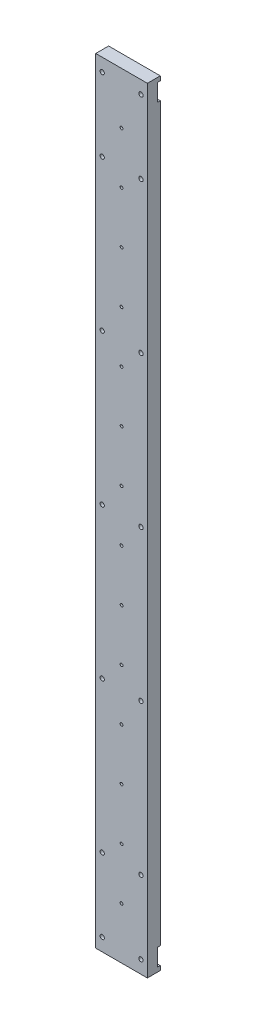
SolidWorks part; units mm, degrees
material "6061 合金"
ref_plane "Front Plane" through (0, 0, 0) normal (0, 0, 1) x (1, 0, 0)
ref_plane "Top Plane" through (0, 0, 0) normal (0, 1, 0) x (1, 0, 0)
ref_plane "Right Plane" through (0, 0, 0) normal (1, 0, 0) x (0, 0, -1)
sketch "Sketch1" plane through (0, 0, 0) normal (0, 0, 1) x (1, 0, 0)
  line L1 (-30, 450) -> (30, 450)
  line L2 (-30, 450) -> (-30, -450)
  line L3 (-30, -450) -> (30, -450)
  line L4 (30, 450) -> (30, -450)
  line L5 (-30, 450) -> (30, -450) construction
  line L6 (-30, -450) -> (30, 450) construction
  point P0 (0, 0)
  dimension "D1" = 60
  dimension "D2" = 900
extrude "Boss-Extrude1" add sketch "Sketch1" along normal blind 15
hole_wizard "CBORE for M6 Hex Socket Head Cap Screw1" positions "Sketch2" profile "Sketch3" counterbore size "M6" standard "ISO"
sketch "Sketch2" plane through (0, 0, 15) normal (0, 0, 1) x (1, 0, 0)
  line L0 (0, 0) -> (176.5363, 0) construction
  point P0 (0, 475)
  point P2 (0, 150)
  point P4 (0, -150)
  point P6 (0, -475)
  dimension "D1" = 300
  dimension "D2" = 950
sketch "Sketch3" plane through (0, 475, 15) normal (1, 0, 0) x (0, -1, 0)
  line L0 (0, 0) -> (0, 15)
  line L1 (0, 15) -> (3.3, 15)
  line L3 (3.3, 15) -> (3.3, 6.4)
  line L4 (3.3, 6.4) -> (5.5, 6.4)
  line L5 (5.5, 6.4) -> (5.5, 0)
  line L7 (5.5, 0) -> (0, 0)
  line L11 (0, -6.35) -> (0, 107.95) construction
  dimension "通孔孔直径" = 6.6
  dimension "通孔孔深度" = 15
  dimension "柱形沉头孔直径" = 11
  dimension "柱形沉头孔深度" = 6.4
sketch "Sketch5" plane through (0, 0, 0) normal (0, 0, -1) x (-1, 0, 0)
  line L0 (-30, -450) -> (-30, 450) construction
  line L1 (-30, 445) -> (30, 445)
  line L2 (-30, 445) -> (-30, 425)
  line L3 (-30, 425) -> (30, 425)
  line L4 (30, 445) -> (30, 425)
  line L5 (30, 450) -> (30, -450) construction
  line L6 (30, -450) -> (-30, -450) construction
  line L7 (-30, -445) -> (30, -445)
  line L8 (-30, -445) -> (-30, -425)
  line L9 (-30, -425) -> (30, -425)
  line L10 (30, -445) -> (30, -425)
  line L11 (-30, 450) -> (30, 450) construction
  dimension "D1" = 20
  dimension "D2" = 5
  dimension "D3" = 5
extrude "Cut-Extrude2" cut sketch "Sketch5" against normal blind 3
sketch "Sketch7" plane through (0, 0, 0) normal (0, 0, -1) x (-1, 0, 0)
  line L0 (-30, 425) -> (30, 425) construction
  line L1 (-7.5, 425) -> (7.5, 425)
  line L2 (-7.5, 425) -> (-7.5, -425)
  line L3 (-7.5, -425) -> (7.5, -425)
  line L4 (7.5, 425) -> (7.5, -425)
  line L5 (30, -425) -> (-30, -425) construction
  dimension "D1" = 15
  dimension "D2" = 7.5
extrude "Cut-Extrude3" cut sketch "Sketch7" against normal blind 2
hole_wizard "M4 Tapped Hole1" positions "Sketch8" profile "Sketch9" tap size "M4" standard "ISO" end condition through all
sketch "Sketch8" plane through (0, 0, 2) normal (0, 0, -1) x (-1, 0, 0)
  line L0 (0, 425) -> (0, 390) construction
  line L1 (7.5, 425) -> (-7.5, 425) construction
  point P0 (0, 390)
  dimension "D1" = 35
sketch "Sketch9" plane through (0, 390, 2) normal (1, 0, 0) x (0, 1, 0)
  line L0 (0, 0) -> (0, 13)
  line L1 (0, 13) -> (1.65, 13)
  line L2 (1.65, 13) -> (1.65, 0)
  line L5 (1.65, 0) -> (0, 0)
  line L11 (0, -6.35) -> (0, 107.95) construction
  dimension "通孔螺纹孔钻头直径" = 3.3
  dimension "通孔螺纹孔钻头深度" = 13
cosmetic thread "Cosmetic Thread1" parameters "D2"=4
pattern_linear "LPattern1" count 14 spacing 60 along (0, -1, 0) of "M4 Tapped Hole1"
cosmetic thread "Cosmetic Thread2" parameters "D2"=4
cosmetic thread "Cosmetic Thread3" parameters "D2"=4
cosmetic thread "Cosmetic Thread4" parameters "D2"=4
cosmetic thread "Cosmetic Thread5" parameters "D2"=4
cosmetic thread "Cosmetic Thread6" parameters "D2"=4
cosmetic thread "Cosmetic Thread7" parameters "D2"=4
cosmetic thread "Cosmetic Thread8" parameters "D2"=4
cosmetic thread "Cosmetic Thread9" parameters "D2"=4
cosmetic thread "Cosmetic Thread10" parameters "D2"=4
cosmetic thread "Cosmetic Thread11" parameters "D2"=4
cosmetic thread "Cosmetic Thread12" parameters "D2"=4
cosmetic thread "Cosmetic Thread13" parameters "D2"=4
cosmetic thread "Cosmetic Thread14" parameters "D2"=4
hole_wizard "M6 Tapped Hole1" positions "Sketch10" profile "Sketch11" tap size "M6" standard "ISO" end condition through all
sketch "Sketch10" plane through (0, 0, 3) normal (0, 0, -1) x (-1, 0, 0)
  line L0 (-30, -435) -> (-22.5, -435) construction
  line L1 (-30, -425) -> (-30, -445) construction
  line L3 (0, -445) -> (0, -434.4677) construction
  line L4 (-30, -445) -> (30, -445) construction
  line L6 (-30, 435) -> (-22.5, 435) construction
  line L7 (-30, 445) -> (-30, 425) construction
  line L9 (0, 445) -> (0, 434.9254) construction
  line L10 (30, 445) -> (-30, 445) construction
  point P0 (-22.5, 435)
  point P2 (22.5, 435)
  point P4 (-22.5, -435)
  point P6 (22.5, -435)
  dimension "D1" = 45
  dimension "D2" = 45
sketch "Sketch11" plane through (22.5, 435, 3) normal (1, 0, 0) x (0, 1, 0)
  line L0 (0, 0) -> (0, 12)
  line L1 (0, 12) -> (2.5, 12)
  line L2 (2.5, 12) -> (2.5, 0)
  line L5 (2.5, 0) -> (0, 0)
  line L11 (0, -6.35) -> (0, 107.95) construction
  dimension "通孔螺纹孔钻头直径" = 5
  dimension "通孔螺纹孔钻头深度" = 12
cosmetic thread "Cosmetic Thread15" parameters "D2"=6
cosmetic thread "Cosmetic Thread16" parameters "D2"=6
cosmetic thread "Cosmetic Thread17" parameters "D2"=6
cosmetic thread "Cosmetic Thread18" parameters "D2"=6
hole_wizard "M6 Tapped Hole2" positions "Sketch12" profile "Sketch13" tap size "M6" standard "ISO" end condition through all
sketch "Sketch12" plane through (0, 0, 15) normal (0, 0, 1) x (1, 0, 0)
  line L0 (0, 0) -> (0, 16.6529) construction
  point P0 (-22.5, 0)
  point P2 (22.5, 0)
  dimension "D1" = 45
sketch "Sketch13" plane through (-22.5, 0, 15) normal (1, 0, 0) x (0, -1, 0)
  line L0 (0, 0) -> (0, 15)
  line L1 (0, 15) -> (2.5, 15)
  line L2 (2.5, 15) -> (2.5, 0)
  line L5 (2.5, 0) -> (0, 0)
  line L11 (0, -6.35) -> (0, 107.95) construction
  dimension "通孔螺纹孔钻头直径" = 5
  dimension "通孔螺纹孔钻头深度" = 15
cosmetic thread "Cosmetic Thread19" parameters "D2"=6
cosmetic thread "Cosmetic Thread20" parameters "D2"=6
pattern_linear "LPattern2" count 3 spacing 175 along (0, -1, 0) count 3 spacing 175 along (0, 1, 0) seed only of "M6 Tapped Hole2"
cosmetic thread "Cosmetic Thread21" parameters "D2"=6
cosmetic thread "Cosmetic Thread22" parameters "D2"=6
cosmetic thread "Cosmetic Thread23" parameters "D2"=6
cosmetic thread "Cosmetic Thread24" parameters "D2"=6
cosmetic thread "Cosmetic Thread25" parameters "D2"=6
cosmetic thread "Cosmetic Thread26" parameters "D2"=6
cosmetic thread "Cosmetic Thread27" parameters "D2"=6
cosmetic thread "Cosmetic Thread28" parameters "D2"=6
